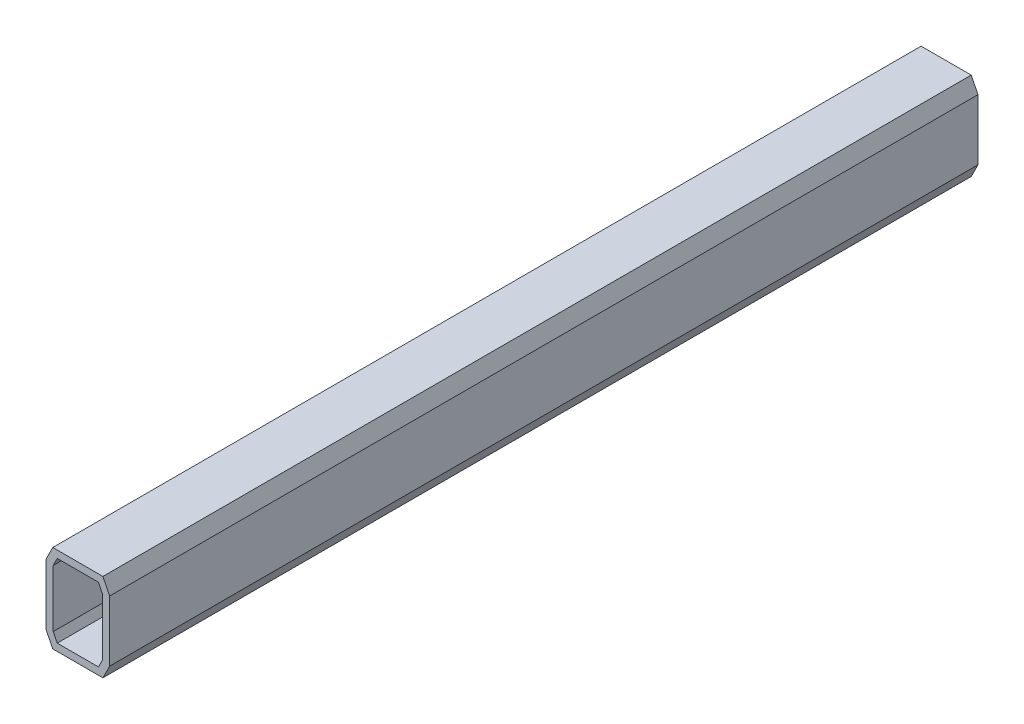
SolidWorks part; units mm, degrees
ref_plane "Front Plane" through (0, 0, 0) normal (0, 0, 1) x (1, 0, 0)
ref_plane "Top Plane" through (0, 0, 0) normal (0, 1, 0) x (1, 0, 0)
ref_plane "Right Plane" through (0, 0, 0) normal (1, 0, 0) x (0, 0, -1)
other "Configuration Table"
sketch "Sketch1" plane through (0, 0, 0) normal (0, 0, 1) x (1, 0, 0)
  line L0 (-17.3197, 136.5) -> (17.3197, 136.5)
  line L3 (17.3197, 136.5) -> (22, 127.1393)
  line L4 (22, 127.1393) -> (22, 85.1607)
  line L5 (22, 85.1607) -> (17.3197, 75.8)
  line L6 (17.3197, 75.8) -> (-17.3197, 75.8)
  line L7 (-17.3197, 75.8) -> (-22, 85.1607)
  line L8 (-22, 85.1607) -> (-22, 127.1393)
  line L9 (-22, 127.1393) -> (-17.3197, 136.5)
  line L10 (-14.2295, 131.5) -> (14.2295, 131.5)
  line L11 (14.2295, 131.5) -> (17, 125.959)
  line L12 (17, 125.959) -> (17, 86.341)
  line L13 (17, 86.341) -> (14.2295, 80.8)
  line L14 (14.2295, 80.8) -> (-14.2295, 80.8)
  line L15 (-14.2295, 80.8) -> (-17, 86.341)
  line L16 (-17, 86.341) -> (-17, 125.959)
  line L17 (-17, 125.959) -> (-14.2295, 131.5)
  dimension "D1" = 5
extrude "Boss-Extrude1" add sketch "Sketch1" along normal blind 600
